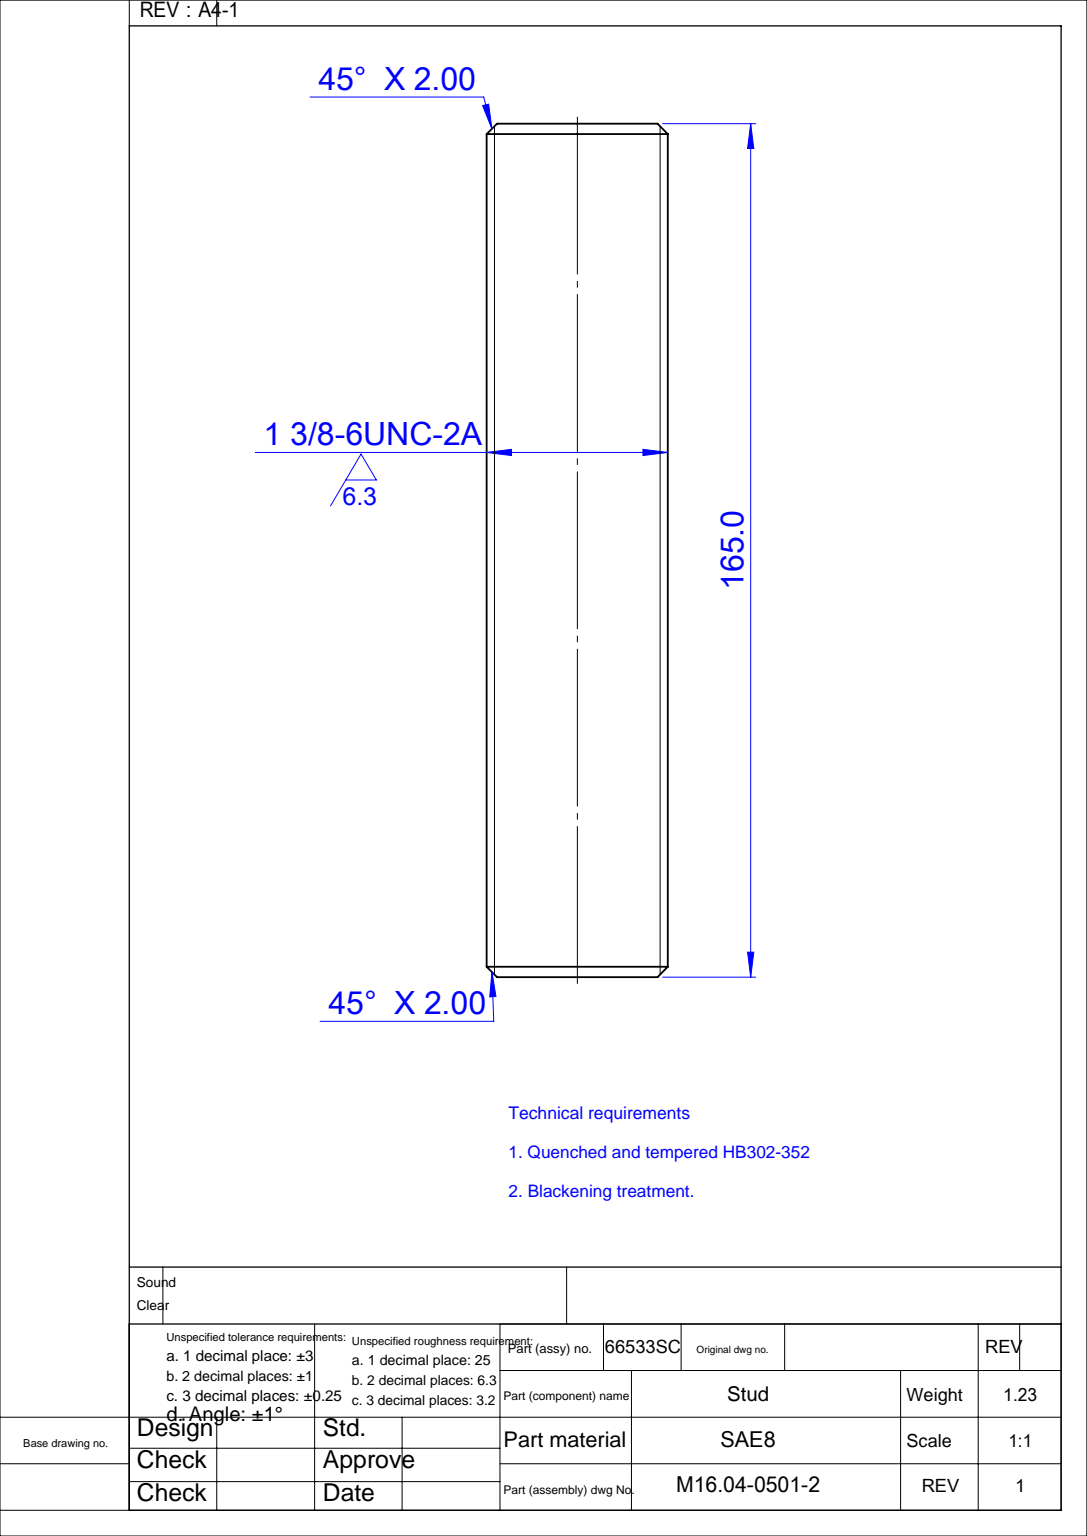
SolidWorks part; units mm, degrees
material "SAE8"
ref_plane "Front Plane" through (0, 0, 0) normal (0, 0, 1) x (1, 0, 0)
ref_plane "Top Plane" through (0, 0, 0) normal (0, 1, 0) x (1, 0, 0)
ref_plane "Right Plane" through (0, 0, 0) normal (1, 0, 0) x (0, 0, -1)
sketch "Sketch1" plane through (0, 0, 0) normal (0, 0, 1) x (1, 0, 0)
  line L0 (0, 158.8607) -> (0, 0) construction
  line L3 (0, 0) -> (-17.5, 0)
  line L4 (0, 0) -> (0, 165)
  line L5 (0, 165) -> (-17.5, 165)
  line L6 (-17.5, 0) -> (-17.5, 165)
  dimension "D1" = 35
  dimension "D2" = 165
revolve "Revolve1" add sketch "Sketch1" angle 360 about L0
cosmetic thread "Cosmetic Thread1" parameters "D2"=32
chamfer "Chamfer1" distance 2 angle 45 2 edges at (0, 0, 17.5) (0, 165, 17.5)
